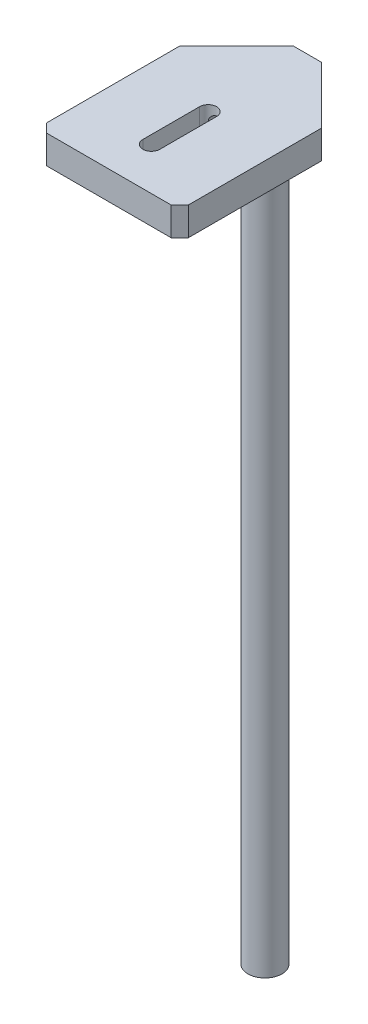
SolidWorks part; units mm, degrees
ref_plane "Front Plane" through (0, 0, 0) normal (0, 0, 1) x (1, 0, 0)
ref_plane "Top Plane" through (0, 0, 0) normal (0, 1, 0) x (1, 0, 0)
ref_plane "Right Plane" through (0, 0, 0) normal (1, 0, 0) x (0, 0, -1)
sketch "Sketch1" plane through (0, 0, 0) normal (0, 1, 0) x (1, 0, 0)
  line L0 (-25, 25) -> (-5, 45)
  line L1 (-25, -25) -> (25, -25)
  line L2 (-25, -25) -> (-25, 25)
  line L4 (25, -25) -> (25, 25)
  line L5 (-25, -25) -> (25, 25) construction
  line L6 (-25, 25) -> (25, -25) construction
  line L7 (-5, 45) -> (5, 45)
  line L8 (5, 45) -> (25, 25)
  point P0 (0, 0)
  dimension "D1" = 50
  dimension "D2" = 50
  dimension "D3" = 70
  dimension "D4" = 10
extrude "Boss-Extrude1" add sketch "Sketch1" along normal blind 10
sketch "Sketch2" plane through (0, 0, 0) normal (0, -1, 0) x (1, 0, 0)
  line L0 (5, -45) -> (-5, -45) construction
  line L1 (0, -45) -> (0, -30) construction
  circle A0 centre (0, -30) radius 6
  dimension "D1" = 12
  dimension "D2" = 15
extrude "Boss-Extrude2" add sketch "Sketch2" along normal blind 260
hole_wizard "M5 Tapped Hole1" positions "Sketch3" profile "Sketch4" tap size "M5" standard "GB"
sketch "Sketch3" plane through (0, 0, -45) normal (0, 0, -1) x (-1, 0, 0)
  line L0 (5, 10) -> (5, 0) construction
  line L1 (-5, 10) -> (5, 10) construction
  point P0 (0, 5)
  dimension "D1" = 5
  dimension "D2" = 5
sketch "Sketch4" plane through (0, 5, -45) normal (1, 0, 0) x (0, 1, 0)
  line L0 (0, 0) -> (0, 38.1618)
  line L1 (0, 38.1618) -> (2.1, 36.9)
  line L2 (2.1, 36.9) -> (2.1, 0)
  line L5 (2.1, 0) -> (0, 0)
  line L10 (0, 38.1618) -> (-2.1, 36.9) construction
  line L11 (0, -6.35) -> (0, 107.95) construction
  dimension "螺纹孔钻头直径" = 4.2
  dimension "螺纹孔钻头深度" = 36.9
  dimension "导头角度" = 118
cosmetic thread "Hole thread line1"
sketch "Sketch5" plane through (0, 0, 0) normal (0, -1, 0) x (1, 0, 0)
  line L0 (0, 10) -> (0, -10) construction
  line L1 (3, 10) -> (3, -10)
  line L2 (-3, 10) -> (-3, -10)
  arc A0 (3, 10) -> (-3, 10) centre (0, 10) ccw
  arc A1 (-3, -10) -> (3, -10) centre (0, -10) ccw
  point P3 (0, 0)
  dimension "D1" = 6
  dimension "D2" = 20
extrude "Cut-Extrude1" cut sketch "Sketch5" against normal through all
chamfer "Chamfer1" distance 3 angle 45 2 edges at (25, 5, 25) (-25, 5, 25)
equation "\"1\"= \"代号代号\""
equation "\"2\"= \"名称代号\""
